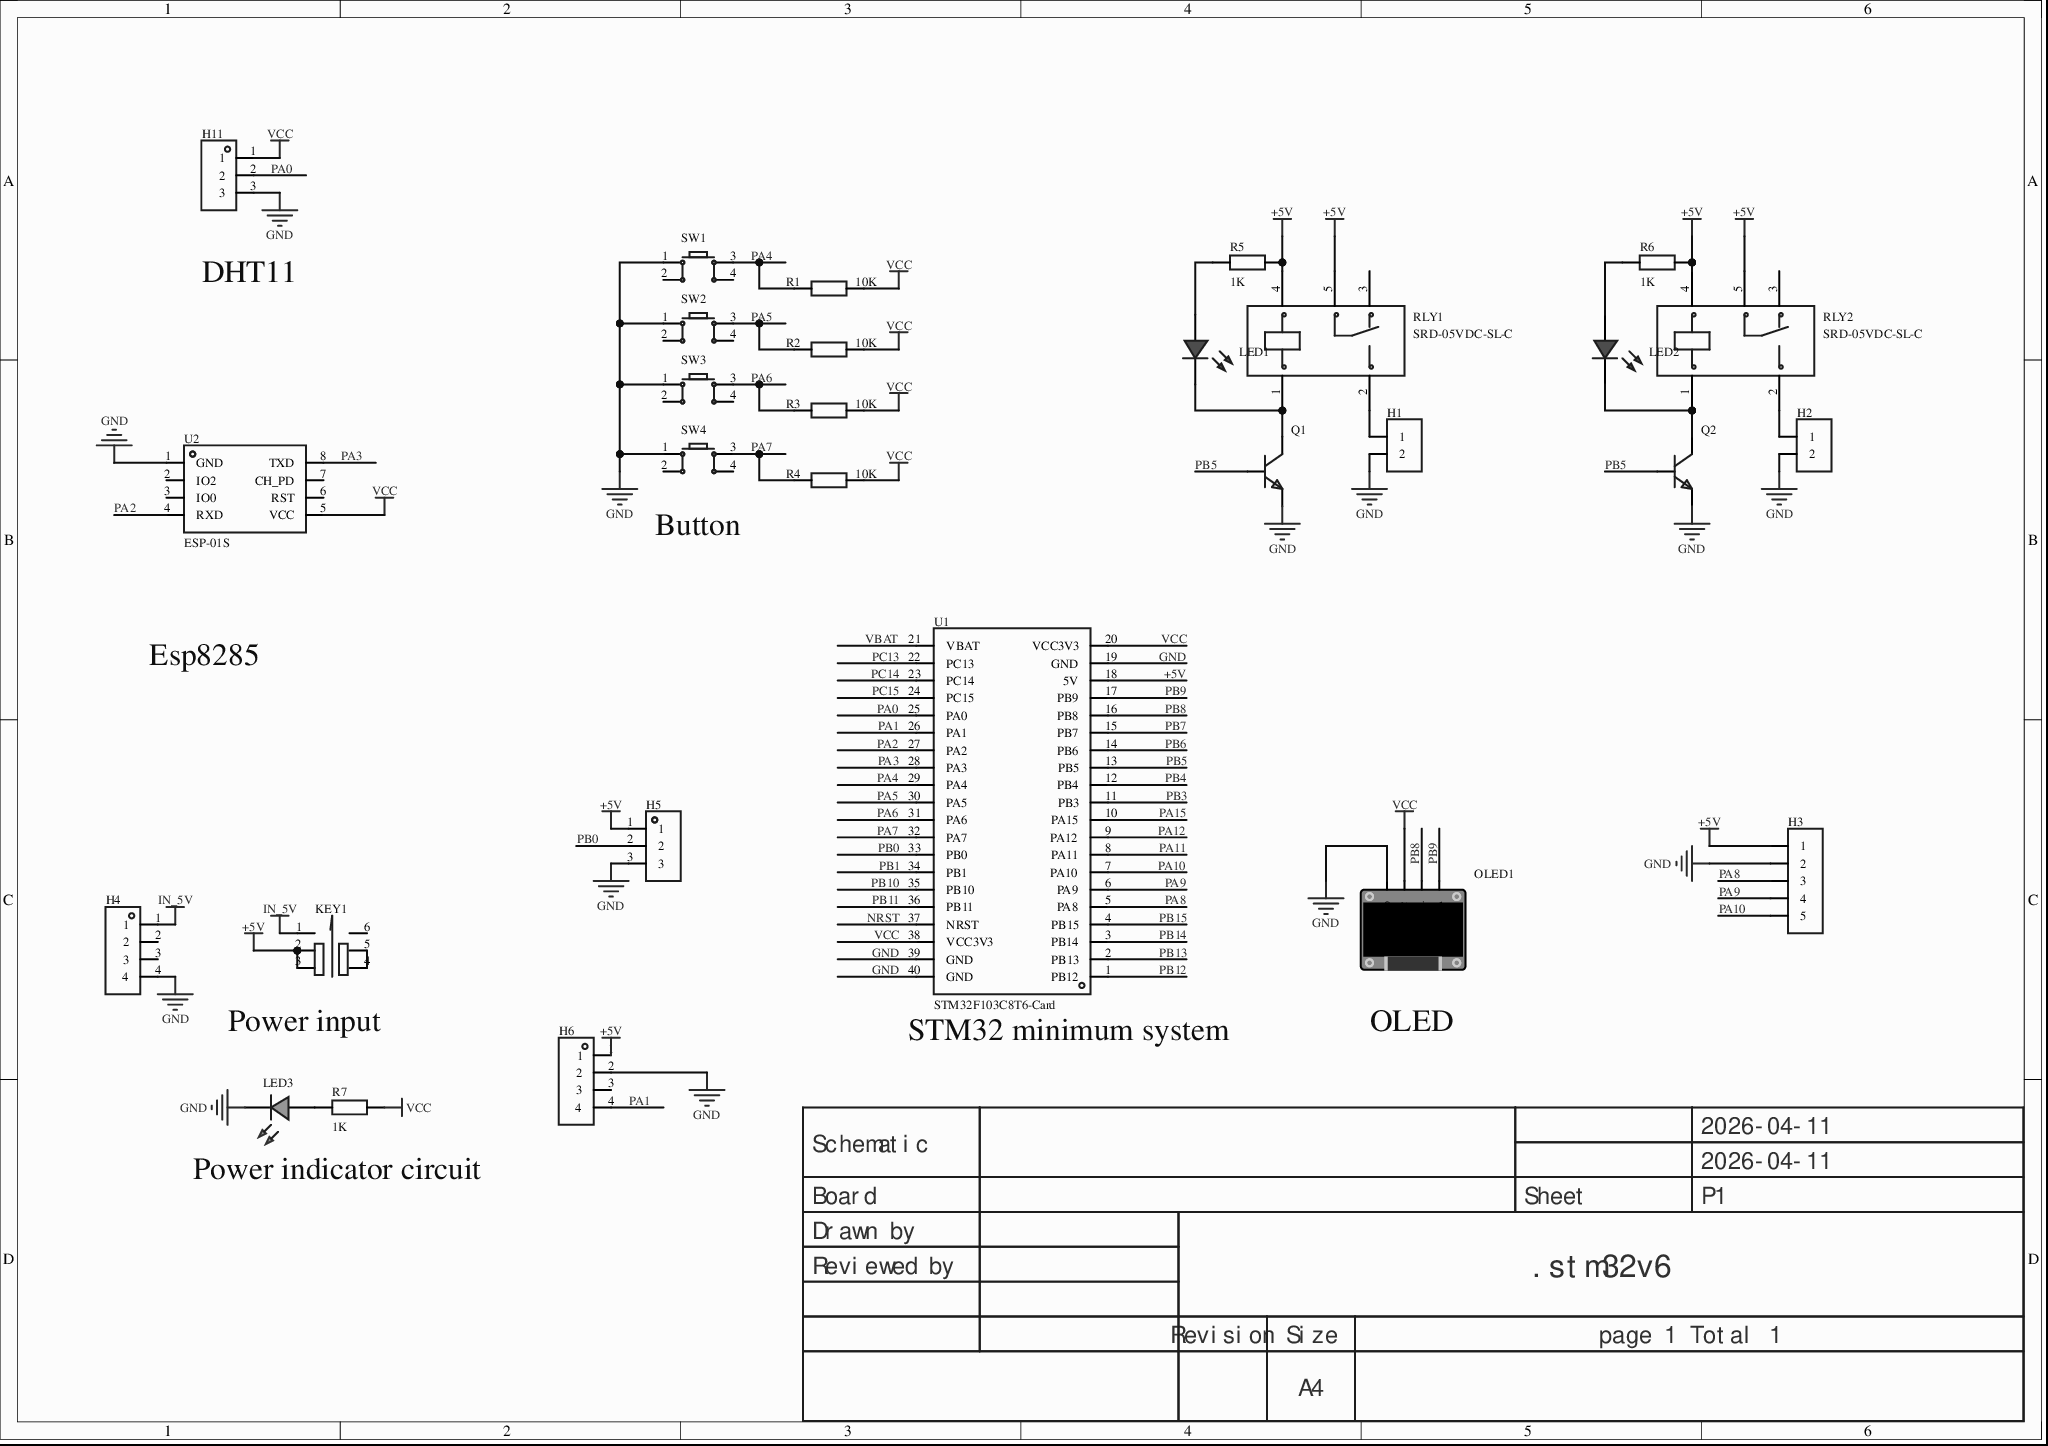
[diagram p0: MISC49853-3.schdoc]
# Altium project MISC49853-2.PrjPcb
1 sheet, 29 parts. Net scope: global (net labels, ports and power ports of the same name join across sheets).
Board file: MISC49853.pcbdoc

## Sheet MISC49853-3.schdoc
size 297 x 209 mm; Version: V1.0; @Project Name: MISC49853; @Page Count: 1; @Update Date: 2026-04-11; @Create Date: 2026-04-11; @Schematic Name: MISC49853; @Page No: 1; @Create Time: 23:22:16; @Update Time: 17:32:40; @Board Name: MISC49853

### Parts
H1  (no value)  [HDR-TH_2P-P2.54-V-F]
H2  (no value)  [HDR-TH_2P-P2.54-V-F]
H3  (no value)  [HDR-TH_5P-P2.54-V-F]
H4  (no value)  [HDR-TH_4P-P2.54-V-F]
H5  (no value)  [HDR-TH_3P-P2.54-V-F]
H6  (no value)  [HDR-TH_4P-P2.54-V-F]
H11  (no value)  [HDR-TH_3P-P2.54-V-F]
KEY1  Self-locking switch 5.8Z white-grey-white 260G  [SW-TH_6P-L5.8-W5.8-P2.00-LS4.5-TR]  (value not drawn)
LED1  (no value)  [LED_TH-3mm]
LED2  (no value)  [LED_TH-3mm]
LED3  (no value)  [LED_TH-3mm]
OLED1  (no value)  [0.96OLED_4P]
Q1  (no value)  [S8050_SOT-23]
Q2  (no value)  [S8050_SOT-23]
R1  10K  [R0603]
R2  10K  [R0603]
R3  10K  [R0603]
R4  10K  [R0603]
R5  1K  [R0603]
R6  1K  [R0603]
R7  1K  [R0603]
RLY1  SRD-05VDC-SL-C  [RELAY-TH_SRD-XXVDC-XL-C]
RLY2  SRD-05VDC-SL-C  [RELAY-TH_SRD-XXVDC-XL-C]
SW1  (no value)  [SW-TH_4P-L6.0-W6.0-P4.50-LS6.5]
SW2  (no value)  [SW-TH_4P-L6.0-W6.0-P4.50-LS6.5]
SW3  (no value)  [SW-TH_4P-L6.0-W6.0-P4.50-LS6.5]
SW4  (no value)  [SW-TH_4P-L6.0-W6.0-P4.50-LS6.5]
U1  STM32F103C8T6-Card  [CONN-TH_L53.3-W22.9_STM32F103C8T6-CARD]
U2  ESP-01S  [WIFIM-TH_ESP-01S]

### Nets
+5V: H3.1 H5.1 H6.1 KEY1.2 KEY1.3 R5.2 R6.2 RLY1.4 RLY1.5 RLY2.4 RLY2.5 U1.18(5V)
GND: H1.2 H2.2 H3.2 H4.4 H5.3 H6.2 H11.3 LED3.2(A) OLED1.1(GND) Q1.2 Q2.2 SW1.1 SW2.1 SW3.1 SW4.1 U1.19(GND) U1.39(GND) U1.40(GND) U2.1(GND)
IN_5V: H4.1 KEY1.1
VCC: H11.1 OLED1.2(VCC) R1.2 R2.2 R3.2 R4.2 R7.2 U1.20(VCC3V3) U1.38(VCC3V3) U2.5(VCC)
NRST: U1.37(NRST)
PA0: H11.2 U1.25(PA0)
PA1: H6.4 U1.26(PA1)
PA2: U1.27(PA2) U2.4(RXD)
PA3: U1.28(PA3) U2.8(TXD)
PA4: R1.1 SW1.3 U1.29(PA4)
PA5: R2.1 SW2.3 U1.30(PA5)
PA6: R3.1 SW3.3 U1.31(PA6)
PA7: R4.1 SW4.3 U1.32(PA7)
PA8: H3.3 U1.5(PA8)
PA9: H3.4 U1.6(PA9)
PA10: H3.5 U1.7(PA10)
PA11: U1.8(PA11)
PA12: U1.9(PA12)
PA15: U1.10(PA15)
PB0: H5.2 U1.33(PB0)
PB1: U1.34(PB1)
PB3: U1.11(PB3)
PB4: U1.12(PB4)
PB5: Q1.1 Q2.1 U1.13(PB5)
PB6: U1.14(PB6)
PB7: U1.15(PB7)
PB8: OLED1.3(SCL) U1.16(PB8)
PB9: OLED1.4(SDA) U1.17(PB9)
PB10: U1.35(PB10)
PB11: U1.36(PB11)
PB12: U1.1(PB12)
PB13: U1.2(PB13)
PB14: U1.3(PB14)
PB15: U1.4(PB15)
PC13: U1.22(PC13)
PC14: U1.23(PC14)
PC15: U1.24(PC15)
VBAT: U1.21(VBAT)
NetH1_1: H1.1 RLY1.2
NetH2_1: H2.1 RLY2.2
NetKEY1_4: KEY1.4 KEY1.5
NetLED1_1: LED1.1(C) R5.1
NetLED1_2: LED1.2(A) Q1.3 RLY1.1
NetLED2_1: LED2.1(C) R6.1
NetLED2_2: LED2.2(A) Q2.3 RLY2.1
NetLED3_1: LED3.1(C) R7.1

Not connected (* = marked no-connect by the designer): H4 2 3; H6 3; KEY1 6; RLY1 3; RLY2 3; SW1 2 4; SW2 2 4; SW3 2 4; SW4 2 4; U2 2(IO2)* 3(IO0)* 6(RST)* 7(CH_PD)*

### Notes on the sheet
- (near H11) DHT11
- (near SW4) Button
- Esp8285
- (near KEY1) Power input
- (near U1) STM32 minimum system
- OLED
- Power indicator circuit
- 2026-04-11
- Schematic
- Board
- Sheet
- P1
- Drawn by
- Reviewed by
- .stm32v6
- Revision
- Size
- A4
- page 1 Total 1

### Library data of the parts
H1 H2 = HDR-F_2.54_1x2P: Symbol: Header-Female-2.54_1x2; ConvertToPcb: yes; ModelId: a9450ef445564560a104363b9aacde4e; ModelName: HDR-TH_2P-P2.54-F-LI-1X2P; ModelTransform: 215.7476,98.425,0,0,0,0,0,0,-129.921; Device: HDR-F_2.54_1x2P; AddInBom: yes; SupplierPart: C49661; Supplier Footprint: 插件; FootprintName: HDR-TH_2P-P2.54-V-F
H3 = HDR-F_2.54_1x5P: Symbol: Header-Female-2.54_1x5; ConvertToPcb: yes; ModelId: f49cb6116a3d45e5a64915bf3e00773f; ModelTransform: 519.684,98.464,0,0,0,0,0,0,-124.016; Device: HDR-F_2.54_1x5P; AddInBom: yes; SupplierPart: C50950; Supplier Footprint: 插件; FootprintName: HDR-TH_5P-P2.54-V-F; ModelName: HDR-TH_5P-P2.54-V-F
H4 = HDR-F_2.54_1x4P: Symbol: 2.54-1*4P female; ConvertToPcb: yes; ModelId: d187812051054f85879fcaa51a310d8e0819f05c4eef4c71ace90d822a990e87; ModelTransform: 419.6842,98.464,0,0,0,0,0,0,-118.11; Device: HDR-F_2.54_1x4P; AddInBom: yes; SupplierPart: C2718488; Supplier Footprint: 插件; FootprintName: HDR-TH_4P-P2.54-V-F; ModelName: HDR-TH_4P-P2.54-V-F
H5 H11 = HDR-F_2.54_1x3P: Symbol: PM254V-11-03-H85; 3D Model: f3b3cc5aae9641bf9e56fc160cef875b; 3D Model Transform: 299.9994,100,0,0,0,0,0,0,-118.11; ConvertToPcb: yes; ModelName: HDR2.54-F-LI-1X3P; Device: HDR-F_2.54_1x3P; Supplier Part: C541850; Supplier Footprint: 插件; AddInBom: yes; FootprintName: HDR-TH_3P-P2.54-V-F
H6 = HDR-F_2.54_1x4P: Symbol: 2.54-1*4P female; 3D Model: d187812051054f85879fcaa51a310d8e0819f05c4eef4c71ace90d822a990e87; 3D Model Transform: 419.6842,98.464,0,0,0,0,0,0,-118.11; ConvertToPcb: yes; Device: HDR-F_2.54_1x4P; Supplier Part: C2718488; Supplier Footprint: 插件; AddInBom: yes; FootprintName: HDR-TH_4P-P2.54-V-F; ModelName: HDR-TH_4P-P2.54-V-F
KEY1 = 自锁开关 5.8Z白灰白260G: 耐温260度; Symbol: Self-locking switch 5.8ZWhite and white260G; AddInBom: yes; ModelId: cd839ddf8c8d4e01911ba601e759d3e90819f05c4eef4c71ace90d822a990e87; ModelTransform: 228.346,228.346,0,0,0,0,0,0,-137.795; Device: Self-locking switch 5.8Z white-grey-white 260G; LCSC Part Name: 自锁开关 5.8Z白灰白 260G  5.8*5.8mm; SupplierPart: C56857; ManufacturerPart: 自锁开关 5.8Z白灰白260G; Supplier Footprint: 插件; JLCPCB Part Class: Extended Part; Supplier: LCSC; ConvertToPcb: yes; FootprintName: SW-TH_6P-L5.8-W5.8-P2.00-LS4.5-TR; ModelName: SW-TH_6P-L5.8-W5.8-P2.00-LS4.5-TR
LED1 LED2 = LED_TH-R_3mm: ConvertToPcb: yes; ModelId: a497c992633541038a38947cdc58012f0819f05c4eef4c71ace90d822a990e87; ModelName: LED-TH-3mm_R; ModelTransform: 141.274,153.327,0,0,0,0,-5.984,0,-137.795; Symbol: LED_TH-R; Device: LED_TH-R_3mm; AddInBom: yes; FootprintName: LED_TH-3mm; Supplier Footprint: 插件
LED3 = LED_TH-G_3mm: AddInBom: yes; ModelId: 07c881668c9448ef9b36eb6a2126ca130819f05c4eef4c71ace90d822a990e87; ModelName: LED-TH-3mm_G; ModelTransform: 141.27444,153.32669525336098,354.32999763315956,0,0,0,-5.90551,0,-137.79528; Symbol: LED_TH-G; Device: LED_TH-G_3mm; ConvertToPcb: yes; FootprintName: LED_TH-3mm; Supplier Footprint: 插件
OLED1 = 0.96OLED模块_4P: Symbol: 0.96OLED module_4P; ConvertToPcb: yes; ModelId: 79c000fdb68d45a296c2e9bedf4f9055; ModelTransform: 1393.69792,1318.895,0,0,0,0,0,-560.079,-137.795; Device: 0.96OLED module_4P; AddInBom: yes; FootprintName: 0.96OLED_4P; Supplier Footprint: 插件; ModelName: 0.96OLED_4P
Q1 Q2 = S8050_SOT_NPN: Symbol: NPN; ConvertToPcb: yes; ModelId: c62791f0466c4ae2a892c056b845b0ca0819f05c4eef4c71ace90d822a990e87; ModelName: SOT-23-3P_L2.9-W1.3-H1.0-LS2.4-P0.95; ModelTransform: 98.6,114.12,41.29,180,0,0,0,0,-3; Device: S8050_SOT_NPN; AddInBom: yes; Supplier Footprint: SOT-23; FootprintName: S8050_SOT-23
R1-R7 = Res_0603: Symbol: Resistor; ConvertToPcb: yes; ModelId: fc143cca1e79419f9cd78b61e9279f080819f05c4eef4c71ace90d822a990e87; ModelTransform: 31.8897,63.7794,0,90,0,0,0,0,0; Device: Res_0603; AddInBom: yes; Supplier Footprint: 0603; FootprintName: R0603; ModelName: R0603
  R1-R4: Value: 10K
  R5-R7: Value: 1K
RLY1 RLY2 = SRD-05VDC-SL-C: Coil voltage:5V;Contact form:One changeover:1C (SPDT);Contact rating (resistive load):-;Max switching voltage:250V@AC;Max switching current:15A;; Manufacturer: 松乐; AddInBom: yes; ModelId: d0eda9b8bf8746d18ae810ab88dc78e70819f05c4eef4c71ace90d822a990e87; ModelName: RELAY-TH_L19.2-W15.6-H15.8; ModelTransform: 755.904,622.4397,0,0,0,0,34.882,0,-118.11; Coil Voltage: 5V; Coil Rated Power: 360mW; Switching Current(Max): 15A; Coil Type: Non-polar, single coil; Coil Resistance: 70Ω; Contact Resistance: 100mΩ; Operate Time: 10ms; Symbol: SRD-05VDC-SL-C; Device: SRD-05VDC-SL-C; LCSC Part Name: 蓝色 单组转换型继电器; SupplierPart: C35449; ManufacturerPart: SRD-05VDC-SL-C; Supplier Footprint: 插件,15.6x19.2mm; JLCPCB Part Class: Extended Part; Datasheet: https://example.com/datasheet/SRD-05VDC-SL-C/36422.html; Supplier: LCSC; ConvertToPcb: yes; FootprintName: RELAY-TH_SRD-XXVDC-XL-C; Contact Form: One changeover: 1C (SPDT); Number of Pins: 5; Contact Rating: -; Switching Voltage(Max): 250V@AC; Release Time: 10ms
SW1-SW4 = Key_TH_6x6x6: Contact current:50mA;Rated voltage(DC):12V;Insulation resistance:100MΩ;Circuit structure:SPST;Mounting:Through-hole;Button shape:Round button;Button/cap colour:Black;Actuating force:260gf@±30gf;Operating temperature:-25℃~+70℃;Pin style:PC pin;Switch length:6mm;Switch width:6mm;Switch height:6mm;With bracket:No;; Symbol: Tact switch; AddInBom: yes; ModelId: 20eee248bc684ccd8cbdbb1d0d91ec6f0819f05c4eef4c71ace90d822a990e87; ModelName: SW-TH_4P-L6.0-W6.0-H5.0-LS6.5-P4.50; ModelTransform: 236.22,323.03,0,90,0,0,0,0,-137.795; Device: Key_TH_6x6x6; ConvertToPcb: yes; FootprintName: SW-TH_4P-L6.0-W6.0-P4.50-LS6.5; Supplier Footprint: 插件
U1 = STM32F103C8T6-Card: AddInBom: yes; Symbol: STM32F103C8T6-CARD; Device: STM32F103C8T6-Card; LCSC Part Name: STM32F103C8T6-Card; SupplierPart: C9900077949; ManufacturerPart: STM32F103C8T6-Card; Supplier Footprint: 插件; Supplier: LCSC; ConvertToPcb: yes; FootprintName: CONN-TH_L53.3-W22.9_STM32F103C8T6-CARD
U2 = ESP-01S_C111009: AddInBom: yes; ModelId: eb7175da78ae48b3b1568cfe3027405f0819f05c4eef4c71ace90d822a990e87; ModelTransform: 582.676,976.37608,0,0,0,0,0,388.346,-118.11; Symbol: ESP-01S; Device: ESP-01S_C111009; LCSC Part Name: ESP-01S; SupplierPart: C111009; ManufacturerPart: ESP-01S; Supplier Footprint: -; JLCPCB Part Class: Extended Part; Supplier: LCSC; ConvertToPcb: yes; FootprintName: WIFIM-TH_ESP-01S; ModelName: WIFIM-TH_ESP-01S